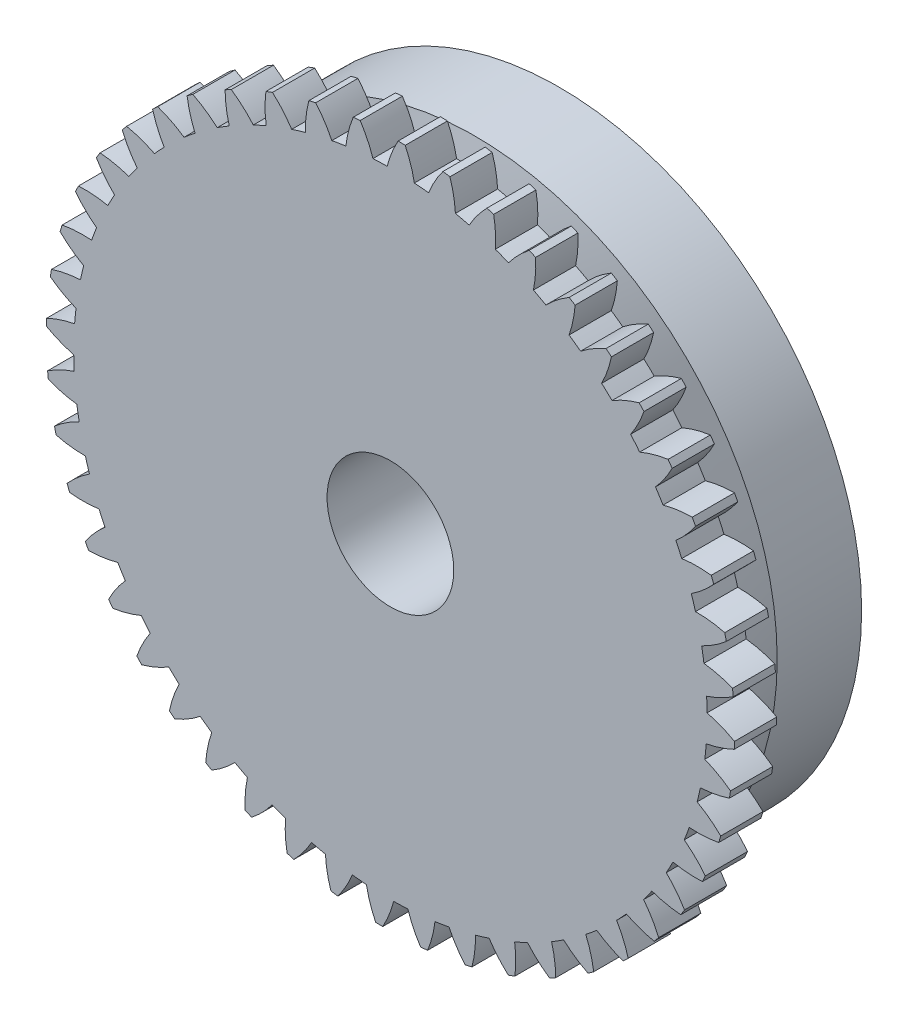
from build123d import *

# Parameters (mm, degrees)
SKETCH1_R           = 7.16
BOSS_EXTRUDE1_DEPTH = 2
SKETCH3_R           = 7.16
SKETCH2_R           = 7.5
SKETCH4_R           = 7.5
BOSS_EXTRUDE2_DEPTH = 1
BOSS_EXTRUDE3_START = -1
BOSS_EXTRUDE3_DEPTH = 1
CIRPATTERN1_COUNT   = 48
SKETCH7_R           = 1.5
CUT_EXTRUDE1_DEPTH  = 5


with BuildPart() as part:
    # Sketch1 → Boss-Extrude1 (new body)
    with BuildSketch(Plane.XY):
        Circle(SKETCH1_R)
    extrude(amount=BOSS_EXTRUDE1_DEPTH)

    # Sketch3 → Loft3 section 0
    with BuildSketch(Plane.XY.offset(2)):
        Circle(SKETCH3_R)
    # Sketch2 → Loft3 section 1
    with BuildSketch(Plane.XY.offset(3)):
        Circle(SKETCH2_R)
    loft()

    # Sketch4 → Boss-Extrude2 (add)
    with BuildSketch(Plane.XY.offset(3)):
        Circle(SKETCH4_R)
    extrude(amount=BOSS_EXTRUDE2_DEPTH)

    # Sketch6 → Boss-Extrude3 (add)
    with BuildSketch(Plane.XY.offset(4).offset(BOSS_EXTRUDE3_START)):
        with BuildLine():
            ThreePointArc((0.349918245, 8.142484708), (0.266660525, 8.145636388), (0.183374937, 8.147936772))
            ThreePointArc((0.183374937, 8.147936772), (0.031553387, 7.832398526), (-0.077350475, 7.499601116))
            ThreePointArc((-0.077350475, 7.499601116), (0.245393121, 7.495984406), (0.567682242, 7.478484932))
            ThreePointArc((0.567682242, 7.478484932), (0.480777544, 7.81769245), (0.349918245, 8.142484708))
        make_face()
    boss_extrude3 = extrude(amount=BOSS_EXTRUDE3_DEPTH)

    # CirPattern1: Boss-Extrude3 ×48 about axis
    cirpattern1_axis = Axis((0, 0, 0), (0, 0, 1))
    for i in range(1, CIRPATTERN1_COUNT):
        add(boss_extrude3.rotate(cirpattern1_axis, i * 360 / CIRPATTERN1_COUNT))

    # Sketch7 → Cut-Extrude1 (cut)
    with BuildSketch(Plane.XY.offset(4)):
        Circle(SKETCH7_R)
    extrude(amount=-CUT_EXTRUDE1_DEPTH, mode=Mode.SUBTRACT)


solid = part.part
